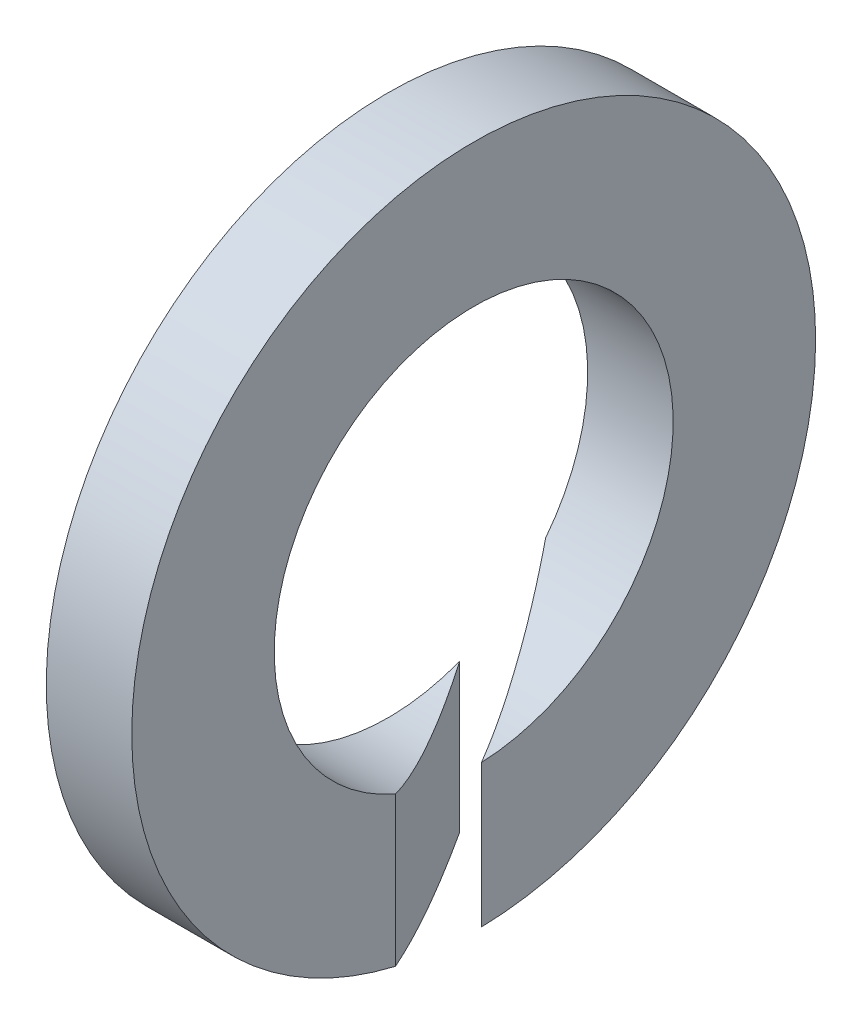
from build123d import *

# Parameters (mm, degrees)
SKETCH1_W          = 3
SKETCH1_H          = 5
CUT_EXTRUDE1_REACH = 24.972


with BuildPart() as part:
    # Sketch1 → Revolve1 (revolve)
    with BuildSketch(Plane.XY, mode=Mode.PRIVATE) as revolve1_sk:
        with Locations((13.982621868, 9.5)):
            Rectangle(SKETCH1_W, SKETCH1_H)
    revolve(revolve1_sk.sketch.rotate(Axis((0, 0, 0), (1, 0, 0)), 90), axis=Axis((0, 0, 0), (1, 0, 0)))

    # Sketch3 → Cut-Extrude1 (cut, up to next)
    with BuildSketch(Plane(origin=(0, 0, 0), x_dir=(1, 0, 0), z_dir=(0, 1, 0)), mode=Mode.PRIVATE) as cut_extrude1_sk1:
        Polygon((7.694741439, 13.902815003), (23.953594269, -14.55017745), (22.65325389, -15.293229095), (5.96980012, 13.902815003), align=None)
    cut_extrude1_tool1 = extrude(cut_extrude1_sk1.sketch, amount=-CUT_EXTRUDE1_REACH, mode=Mode.PRIVATE) & part.part
    add(cut_extrude1_tool1.solids().sort_by_distance((15.064598, 0, 0.510242))[0], mode=Mode.SUBTRACT)


solid = part.part
